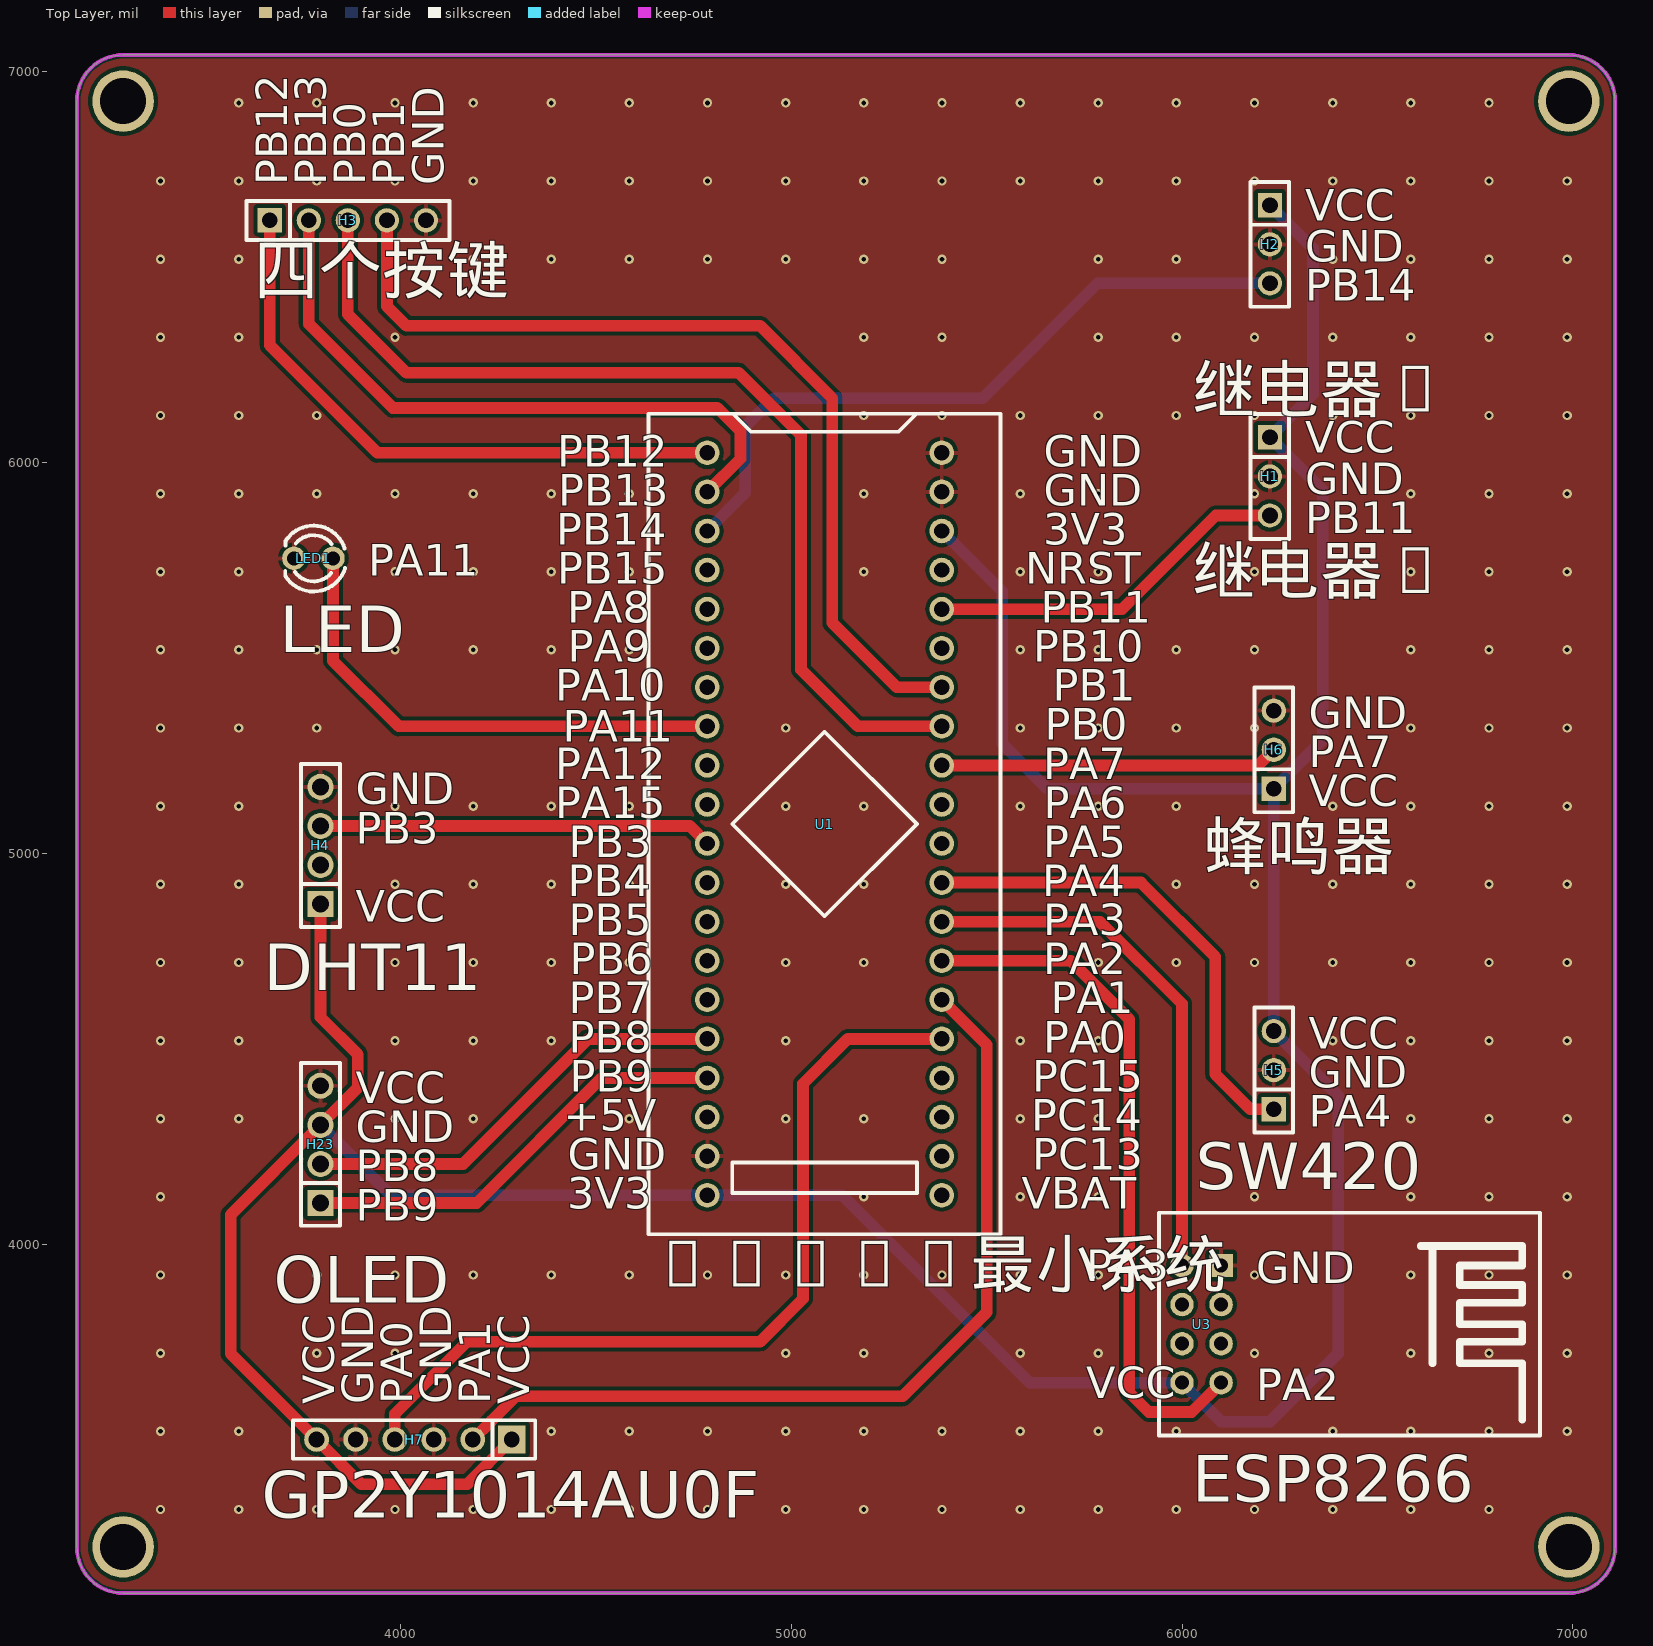
[diagram p0: Top Layer view]
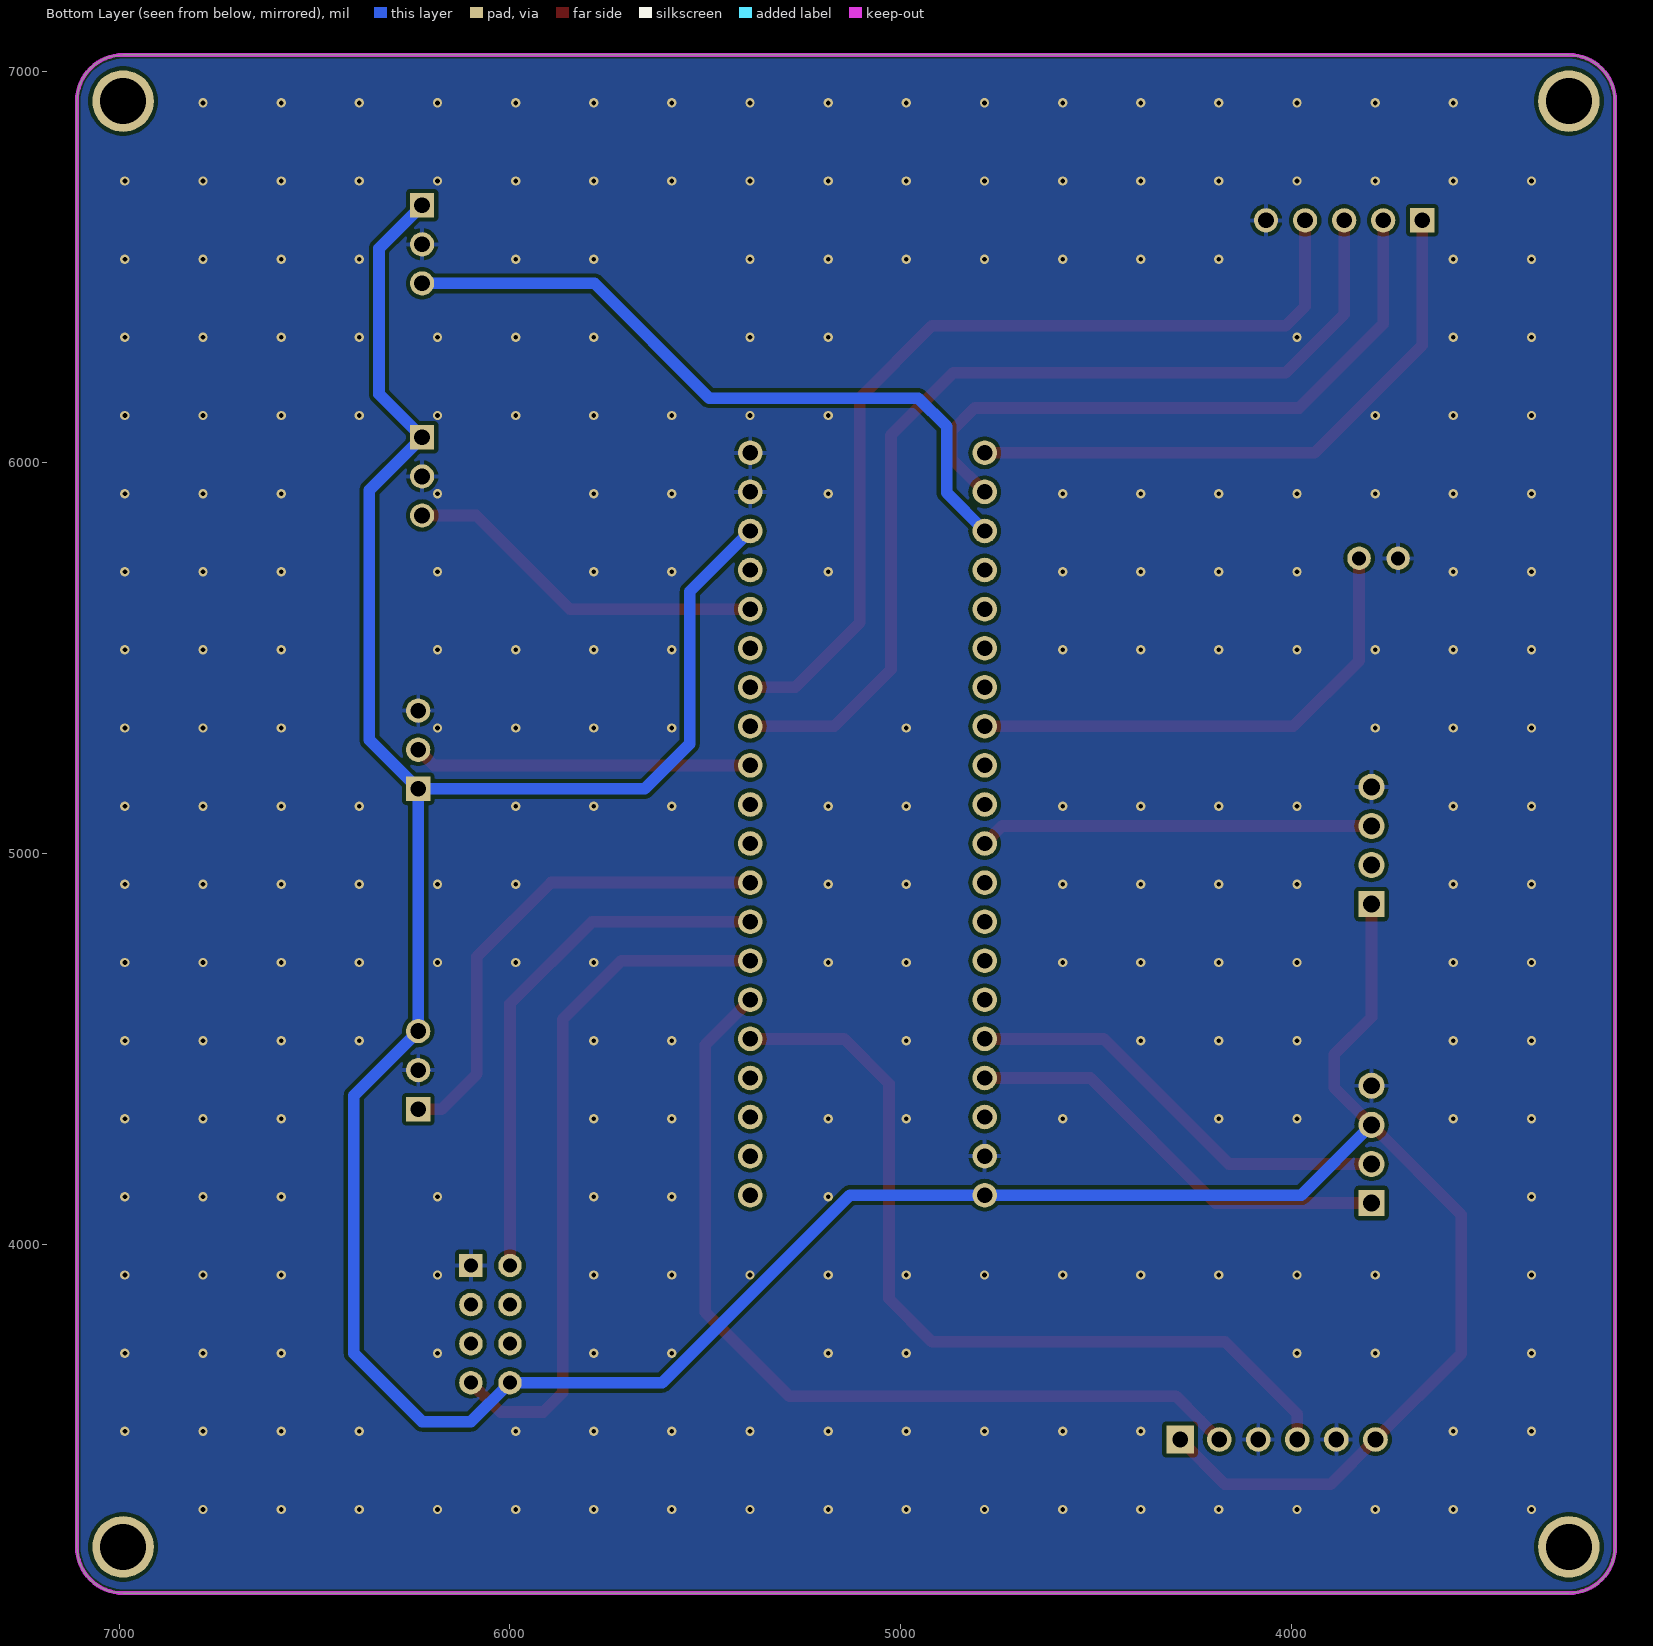
[diagram p1: Bottom Layer view, seen from below]
# Altium PCB MISC51358.pcbdoc
Units mil, origin at the board's own origin, x right, y up, seen from the top; angles counter-clockwise.
Board outline 3937.01 x 3937.01 mil, 2 copper layers (Top Layer, Bottom Layer), stack 62.206 mil thick; 11 components, 37 nets, 85 pads, 264 vias.

## Layer stack, top to bottom
Top Solder Mask Layer: solder mask 0.394, Dk 3.3
Top Layer: signal copper 1.379
Dielectric1: surface 59.449, FR4, Dk 4.5
Bottom Layer: signal copper 1.378
Bottom Solder Mask Layer: solder mask 0.394, Dk 3.3

## Board outline
6990.39,3106.5 ccw(c6990.39,3224.61) 7108.5,3224.61 7108.5,6925.39 ccw(c6990.39,6925.39) 6990.39,7043.5 3289.61,7043.5 ccw(c3289.61,6925.39) 3171.5,6925.39 3171.5,3224.61 ccw(c3289.61,3224.61) 3289.61,3106.5

## Design rules (kind name [scope] priority, off if disabled: settings)
BoardOutlineClearance copperThickness2oz_1 [All] p2 off: genericclearance=7.99 ignorepadtopadclearanceinfootprint=FALSE except(0: Arc-SplitContinuation Track-SplitContinuation SMDPad-SplitContinuation THPad-SplitContinuation Via-SplitContinuation Fill-SplitContinuation Region-SplitContinuation Poly-SplitContinuation Text-SplitContinuation Hole-SplitContinuation; 5.98: Arc-CutoutEdge Track-CutoutEdge SMDPad-CutoutEdge THPad-CutoutEdge Via-CutoutEdge Text-CutoutEdge; 6.89: Hole-OutlineEdge Hole-CutoutEdge; 10: Poly-OutlineEdge Poly-CutoutEdge; 11.81: Arc-OutlineEdge Track-OutlineEdge SMDPad-OutlineEdge THPad-OutlineEdge Via-OutlineEdge Fill-OutlineEdge Region-OutlineEdge Text-OutlineEdge Fill-CutoutEdge Region-CutoutEdge)
BoardOutlineClearance Plane_innerPlane_1 [All] p4 off: genericclearance=4.02 ignorepadtopadclearanceinfootprint=FALSE except(0: Arc-SplitContinuation Track-SplitContinuation SMDPad-SplitContinuation THPad-SplitContinuation Via-SplitContinuation Fill-SplitContinuation Region-SplitContinuation Poly-SplitContinuation Text-SplitContinuation Hole-SplitContinuation; 5.98: Arc-CutoutEdge Track-CutoutEdge SMDPad-CutoutEdge THPad-CutoutEdge Via-CutoutEdge Text-CutoutEdge; 6.89: Hole-OutlineEdge Hole-CutoutEdge; 10: Poly-OutlineEdge Poly-CutoutEdge; 11.81: Arc-OutlineEdge Track-OutlineEdge SMDPad-OutlineEdge THPad-OutlineEdge Via-OutlineEdge Fill-OutlineEdge Region-OutlineEdge Text-OutlineEdge Fill-CutoutEdge Region-CutoutEdge)
BoardOutlineClearance Copper_copperRegion_1 [All] p6 off: genericclearance=4.02 ignorepadtopadclearanceinfootprint=FALSE except(0: Arc-SplitContinuation Track-SplitContinuation SMDPad-SplitContinuation THPad-SplitContinuation Via-SplitContinuation Fill-SplitContinuation Region-SplitContinuation Poly-SplitContinuation Text-SplitContinuation Hole-SplitContinuation; 5.98: Arc-CutoutEdge Track-CutoutEdge SMDPad-CutoutEdge THPad-CutoutEdge Via-CutoutEdge Text-CutoutEdge; 6.89: Hole-OutlineEdge Hole-CutoutEdge; 10: Poly-OutlineEdge Poly-CutoutEdge; 11.81: Arc-OutlineEdge Track-OutlineEdge SMDPad-OutlineEdge THPad-OutlineEdge Via-OutlineEdge Fill-OutlineEdge Region-OutlineEdge Text-OutlineEdge Fill-CutoutEdge Region-CutoutEdge)
BoardOutlineClearance copperThickness1oz_1 [All] p8: genericclearance=4.02 ignorepadtopadclearanceinfootprint=FALSE except(0: Arc-SplitContinuation Track-SplitContinuation SMDPad-SplitContinuation THPad-SplitContinuation Via-SplitContinuation Fill-SplitContinuation Region-SplitContinuation Poly-SplitContinuation Text-SplitContinuation Hole-SplitContinuation; 5.98: Arc-CutoutEdge Track-CutoutEdge SMDPad-CutoutEdge THPad-CutoutEdge Via-CutoutEdge Text-CutoutEdge; 6.89: Hole-OutlineEdge Hole-CutoutEdge; 10: Poly-OutlineEdge Poly-CutoutEdge; 11.81: Arc-OutlineEdge Track-OutlineEdge SMDPad-OutlineEdge THPad-OutlineEdge Via-OutlineEdge Fill-OutlineEdge Region-OutlineEdge Text-OutlineEdge Fill-CutoutEdge Region-CutoutEdge)
Clearance copperThickness2oz [All] p1 off: gap=7.99 ignorepadtopadclearanceinfootprint=FALSE except(5.98: SMDPad-Track SMDPad-SMDPad THPad-Track SMDPad-THPad THPad-THPad Track-Via SMDPad-Via THPad-Via Via-Via Fill-SMDPad Region-SMDPad Fill-THPad Region-THPad Fill-Via Region-Via Fill-Fill Fill-Region Region-Region Arc-Track Arc-SMDPad Arc-THPad Arc-Via Fill-Arc Region-Arc Arc-Arc Text-Track SMDPad-Text Text-THPad Text-Via Fill-Text Region-Text Arc-Text Text-Text; 6.89: Hole-Track Hole-SMDPad Hole-THPad Hole-Via Fill-Hole Region-Hole Hole-Arc Hole-Text; 10: Poly-Track Poly-SMDPad Poly-THPad Poly-Via Poly-Fill Poly-Region Poly-Poly Poly-Arc Poly-Text Poly-Hole; 11.81: Fill-Track Region-Track)
Clearance Plane_innerPlane [All] p3 off: gap=4.02 ignorepadtopadclearanceinfootprint=FALSE except(5.98: SMDPad-Track SMDPad-SMDPad THPad-Track SMDPad-THPad THPad-THPad Track-Via SMDPad-Via THPad-Via Via-Via Fill-SMDPad Region-SMDPad Fill-THPad Region-THPad Fill-Via Region-Via Fill-Fill Fill-Region Region-Region Arc-Track Arc-SMDPad Arc-THPad Arc-Via Fill-Arc Region-Arc Arc-Arc Text-Track SMDPad-Text Text-THPad Text-Via Fill-Text Region-Text Arc-Text Text-Text; 6.89: Hole-Track Hole-SMDPad Hole-THPad Hole-Via Fill-Hole Region-Hole Hole-Arc Hole-Text; 10: Poly-Track Poly-SMDPad Poly-THPad Poly-Via Poly-Fill Poly-Region Poly-Poly Poly-Arc Poly-Text Poly-Hole; 11.81: Fill-Track Region-Track)
Clearance Copper_copperRegion [All] p5 off: gap=4.02 ignorepadtopadclearanceinfootprint=FALSE except(5.98: SMDPad-Track SMDPad-SMDPad THPad-Track SMDPad-THPad THPad-THPad Track-Via SMDPad-Via THPad-Via Via-Via Fill-SMDPad Region-SMDPad Fill-THPad Region-THPad Fill-Via Region-Via Fill-Fill Fill-Region Region-Region Arc-Track Arc-SMDPad Arc-THPad Arc-Via Fill-Arc Region-Arc Arc-Arc Text-Track SMDPad-Text Text-THPad Text-Via Fill-Text Region-Text Arc-Text Text-Text; 6.89: Hole-Track Hole-SMDPad Hole-THPad Hole-Via Fill-Hole Region-Hole Hole-Arc Hole-Text; 10: Poly-Track Poly-SMDPad Poly-THPad Poly-Via Poly-Fill Poly-Region Poly-Poly Poly-Arc Poly-Text Poly-Hole; 11.81: Fill-Track Region-Track)
Clearance copperThickness1oz [All] p7: gap=4.02 ignorepadtopadclearanceinfootprint=FALSE except(5.98: SMDPad-Track SMDPad-SMDPad THPad-Track SMDPad-THPad THPad-THPad Track-Via SMDPad-Via THPad-Via Via-Via Fill-SMDPad Region-SMDPad Fill-THPad Region-THPad Fill-Via Region-Via Fill-Fill Fill-Region Region-Region Arc-Track Arc-SMDPad Arc-THPad Arc-Via Fill-Arc Region-Arc Arc-Arc Text-Track SMDPad-Text Text-THPad Text-Via Fill-Text Region-Text Arc-Text Text-Text; 6.89: Hole-Track Hole-SMDPad Hole-THPad Hole-Via Fill-Hole Region-Hole Hole-Arc Hole-Text; 10: Poly-Track Poly-SMDPad Poly-THPad Poly-Via Poly-Fill Poly-Region Poly-Poly Poly-Arc Poly-Text Poly-Hole; 11.81: Fill-Track Region-Track)
DiffPairsRouting differentialPair [All] p1: maxlimit=6 minlimit=6 mostfreqgap=6 toplayer_minwidth=5 toplayer_prefwidth=10 toplayer_maxwidth=100 toplayer_mingap=6 toplayer_prefgap=6 toplayer_maxgap=6 bottomlayer_minwidth=5 bottomlayer_prefwidth=10 bottomlayer_maxwidth=100 bottomlayer_mingap=6 bottomlayer_prefgap=6 bottomlayer_maxgap=6 maxuncoupledlength=10
HoleToHoleClearance otherClearance [All] p1: gap=11.81 allowstackedmicrovias=TRUE
Length netLength [All] p1: minlimit=0 maxlimit=0
PasteMaskExpansion pasteMaskExpansion [All] p1: expansion=0
PlaneConnect innerPlane [All] p1: planeconnectstyle=Relief reliefexpansion=20 reliefentries=4 reliefconductorwidth=10 reliefairgap=10
PolygonConnect copperRegion [All] p1: connectstyle=Relief reliefconductorwidth=10 reliefentries=4 polygonreliefangle="90 Angle" airgapwidth=10 via.connectstyle=Relief via.reliefconductorwidth=10 via.reliefentries=4 via.polygonreliefangle="90 Angle" via.airgapwidth=10
RoutingVias viaSize [All] p1: holewidth=12.01 width=24.02 viastyle="Through Hole" minholewidth=11.81 minwidth=19.68 maxholewidth=248.03 maxwidth=393.7
SolderMaskExpansion solderMaskExpansion [IsVia] p1: expansion=-1000 istentingtop=TRUE
SolderMaskExpansion solderMaskExpansion [All] p2: expansion=2.01 istentingtop=FALSE
Width copperThickness2oz_2 [All] p1 off: maxlimit=100 minlimit=8 preferedwidth=10
Width copperThickness1oz_2 [All] p2: maxlimit=100 minlimit=5 preferedwidth=30

## Components (designator, comment, footprint, x,y, rotation, side; value= is the part's Value field where it differs from the comment)
H1 "" HDR-TH_3P-P2.54-V-F 6225,5964.59 r270 top
H2 "" HDR-TH_3P-P2.54-V-F 6225,6558.68 r270 top
H3 "" HDR-TH_5P-P2.54-V-F 3865,6620 r0 top
H4 "" HDR-TH_4P-P2.54-V-F 3795,5020 r90 top
H5 "" HDR-TH_3P-P2.54-V-F 6234.84,4445 r90 top
H6 "" HDR-TH_3P-P2.54-V-F 6234.84,5265.03 r90 top
H7 "" HDR-TH_6P-P2.54-V-F 4034.9,3499.62 r180 top
H23 "" HDR-TH_4P-P2.54-V-F 3795,4255 r90 top
LED1 "" LED_TH-3mm 3776.87,5755 r180 top
U1 "STM32F103C8T6-Card" CONN-TH_L53.3-W22.9_STM32F103C8T6-CARD 5085,5075 r270 top
U3 "ESP8266-01S" WIFIM-TH_ESP8266-01S 6050,3795 r270 top

## Footprints (in the part's own frame and the unit in brackets; to place one, negate y for a bottom-side part, rotate by r counter-clockwise, add the part's x,y. Pads: shape width x height; smd on the part's side, far side on the other; paste and mask are expansions set on the pad)
CONN-TH_L53.3-W22.9_STM32F103C8T6-CARD [mm]
  round 1.6 hole 1: 1(-24.13,-7.62) 2(-21.59,-7.62) 3(-19.05,-7.62) 4(-16.51,-7.62) 5(-13.97,-7.62) 6(-11.43,-7.62) 7(-8.89,-7.62) 8(-6.35,-7.62) 9(-3.81,-7.62) 10(-1.27,-7.62) 11(1.27,-7.62) 12(3.81,-7.62) 13(6.35,-7.62) 14(8.89,-7.62) 15(11.43,-7.62) 16(13.97,-7.62) 17(16.51,-7.62) 18(19.05,-7.62) 19(21.59,-7.62) 20(24.13,-7.62) 21(24.13,7.62) 22(21.59,7.62) 23(19.05,7.62) 24(16.51,7.62) 25(13.97,7.62) 26(11.43,7.62) 27(8.89,7.62) 28(6.35,7.62) 29(3.81,7.62) 30(1.27,7.62) 31(-1.27,7.62) 32(-3.81,7.62) 33(-6.35,7.62) 34(-8.89,7.62) 35(-11.43,7.62) 36(-13.97,7.62) 37(-16.51,7.62) 38(-19.05,7.62) 39(-21.59,7.62) 40(-24.13,7.62)
  silkscreen extent -26.67,-11.43 26.67,11.43
HDR-TH_3P-P2.54-V-F [mil]
  rect 62x62 hole 40.16: 1(-100,0)
  round 62 hole 40.16: 2(0,0) 3(100,0)
  silkscreen extent -160,-49 160,49
HDR-TH_4P-P2.54-V-F [mm]
  rect 1.7x1.7 hole 1.1: 1(-3.81,0)
  round 1.7 hole 1.1: 2(-1.27,0) 3(1.27,0) 4(3.81,0)
  silkscreen extent -5.29,-1.27 5.29,1.27
HDR-TH_5P-P2.54-V-F [mil]
  rect 62x62 hole 40.16: 1(-200,0)
  round 62 hole 40.16: 2(-100,0) 3(0,0) 4(100,0) 5(200,0)
  silkscreen extent -260,-50 260,50
HDR-TH_6P-P2.54-V-F [mm]
  rect 1.8x1.8 hole 1.02: 1(-6.35,0)
  round 1.6 hole 1.02: 2(-3.81,0) 3(-1.27,0) 4(1.27,0) 5(3.81,0) 6(6.35,0)
  silkscreen extent -7.87,-1.25 7.87,1.25
LED_TH-3mm [mil]
  round 60 hole 36 paste+0 mask+2: 1(-50,0) 2(50,0)
  silkscreen extent -81,-84 72,85
WIFIM-TH_ESP8266-01S [mil]
  rect 60x60 hole 36 paste+0 mask+1.97: 1(-150,50)
  round 60 hole 36 paste+0 mask+1.97: 2(-50,50) 3(50,50) 4(150,50) 5(-150,-50) 6(-50,-50) 7(50,-50) 8(150,-50)
  silkscreen extent -285,-109 285,866

## Free pads (board coordinates)
  round 157.48 hole 118.11: 1(3289.61,6925.39) 1(3289.61,3224.61) 1(6990.39,6925.39) 1(6990.39,3224.61)

## Via types
v1: diameter 24.02, hole 12, Top Layer to Bottom Layer, 264 vias

## Nets (pads, with @x,y where several pads share a name; then routed paths per layer and width w, separated by ;. In a path a pad name is that pad's centre, name@x,y a point inside that pad or via, vN(x,y) a via of type N, cw(c..) or ccw(c..) an arc to the next point about the centre after c; other vN are vias at no path point)
+5V: U1.18
GND: H1.2 H2.2 H3.5 H4.4 H5.2 H6.3 H7.3 H7.5 H23.4 LED1.2 U1.19 U1.39 U1.40 U3.1
  other v1: 3385.6,3320.6 3585.6,3320.6 3785.6,3320.6 3985.6,3320.6 4185.6,3320.6 4385.6,3320.6 4585.6,3320.6 4785.6,3320.6 4985.6,3320.6 5185.6,3320.6 5385.6,3320.6 5585.6,3320.6 5785.6,3320.6 5985.6,3320.6 6185.6,3320.6 6385.6,3320.6 6585.6,3320.6 6785.6,3320.6 3385.6,3520.6 3585.6,3520.6 4385.6,3520.6 4585.6,3520.6 4785.6,3520.6 4985.6,3520.6 5185.6,3520.6 5385.6,3520.6 5585.6,3520.6 5785.6,3520.6 5985.6,3520.6 6385.6,3520.6 6585.6,3520.6 6785.6,3520.6 6985.6,3520.6 3385.6,3720.6 3785.6,3720.6 3985.6,3720.6 4985.6,3720.6 5185.6,3720.6 5585.6,3720.6 5785.6,3720.6 6185.6,3720.6 6585.6,3720.6 6785.6,3720.6 6985.6,3720.6 3385.6,3920.6 3785.6,3920.6 3985.6,3920.6 4185.6,3920.6 4385.6,3920.6 4585.6,3920.6 4785.6,3920.6 4985.6,3920.6 5185.6,3920.6 5385.6,3920.6 5585.6,3920.6 5785.6,3920.6 6185.6,3920.6 6585.6,3920.6 6785.6,3920.6 6985.6,3920.6 3385.6,4120.6 5185.6,4120.6 5585.6,4120.6 5785.6,4120.6 6185.6,4120.6 6585.6,4120.6 6785.6,4120.6 6985.6,4120.6 3385.6,4320.6 3585.6,4320.6 3985.6,4320.6 4185.6,4320.6 4585.6,4320.6 4985.6,4320.6 5185.6,4320.6 5585.6,4320.6 5785.6,4320.6 6585.6,4320.6 6785.6,4320.6 6985.6,4320.6 3385.6,4520.6 3585.6,4520.6 3985.6,4520.6 4185.6,4520.6 4385.6,4520.6 4985.6,4520.6 5585.6,4520.6 5785.6,4520.6 6385.6,4520.6 6585.6,4520.6 6785.6,4520.6 6985.6,4520.6 3385.6,4720.6 3585.6,4720.6 3985.6,4720.6 4185.6,4720.6 4385.6,4720.6 4585.6,4720.6 4985.6,4720.6 5185.6,4720.6 5785.6,4720.6 5985.6,4720.6 6185.6,4720.6 6385.6,4720.6 6585.6,4720.6 6785.6,4720.6 6985.6,4720.6 3385.6,4920.6 3585.6,4920.6 3985.6,4920.6 4185.6,4920.6 4385.6,4920.6 4585.6,4920.6 4985.6,4920.6 5185.6,4920.6 5985.6,4920.6 6185.6,4920.6 6385.6,4920.6 6585.6,4920.6 6785.6,4920.6 6985.6,4920.6 3385.6,5120.6 3585.6,5120.6 3985.6,5120.6 4185.6,5120.6 4385.6,5120.6 4585.6,5120.6 4985.6,5120.6 5185.6,5120.6 5585.6,5120.6 5785.6,5120.6 5985.6,5120.6 6385.6,5120.6 6585.6,5120.6 6785.6,5120.6 6985.6,5120.6 3385.6,5320.6 3585.6,5320.6 3785.6,5320.6 4985.6,5320.6 5585.6,5320.6 5785.6,5320.6 5985.6,5320.6 6185.6,5320.6 6585.6,5320.6 6785.6,5320.6 6985.6,5320.6 3385.6,5520.6 3585.6,5520.6 3785.6,5520.6 3985.6,5520.6 4185.6,5520.6 4385.6,5520.6 4585.6,5520.6 5585.6,5520.6 5785.6,5520.6 5985.6,5520.6 6185.6,5520.6 6585.6,5520.6 6785.6,5520.6 6985.6,5520.6 3385.6,5720.6 3585.6,5720.6 3985.6,5720.6 4185.6,5720.6 4385.6,5720.6 4585.6,5720.6 5185.6,5720.6 5585.6,5720.6 5785.6,5720.6 6185.6,5720.6 6585.6,5720.6 6785.6,5720.6 6985.6,5720.6 3385.6,5920.6 3585.6,5920.6 3785.6,5920.6 3985.6,5920.6 4185.6,5920.6 4385.6,5920.6 4585.6,5920.6 5185.6,5920.6 5585.6,5920.6 5785.6,5920.6 6185.6,5920.6 6585.6,5920.6 6785.6,5920.6 6985.6,5920.6 3385.6,6120.6 3585.6,6120.6 3785.6,6120.6 5185.6,6120.6 5385.6,6120.6 5585.6,6120.6 5785.6,6120.6 5985.6,6120.6 6185.6,6120.6 6385.6,6120.6 6585.6,6120.6 6785.6,6120.6 6985.6,6120.6 3385.6,6320.6 3585.6,6320.6 3985.6,6320.6 5185.6,6320.6 5385.6,6320.6 5785.6,6320.6 5985.6,6320.6 6185.6,6320.6 6385.6,6320.6 6585.6,6320.6 6785.6,6320.6 6985.6,6320.6 3385.6,6520.6 3585.6,6520.6 4185.6,6520.6 4385.6,6520.6 4585.6,6520.6 4785.6,6520.6 4985.6,6520.6 5185.6,6520.6 5385.6,6520.6 5785.6,6520.6 5985.6,6520.6 6385.6,6520.6 6585.6,6520.6 6785.6,6520.6 6985.6,6520.6 3385.6,6720.6 3585.6,6720.6 3785.6,6720.6 3985.6,6720.6 4185.6,6720.6 4385.6,6720.6 4585.6,6720.6 4785.6,6720.6 4985.6,6720.6 5185.6,6720.6 5385.6,6720.6 5585.6,6720.6 5785.6,6720.6 5985.6,6720.6 6185.6,6720.6 6385.6,6720.6 6585.6,6720.6 6785.6,6720.6 6985.6,6720.6 3585.6,6920.6 3785.6,6920.6 3985.6,6920.6 4185.6,6920.6 4385.6,6920.6 4585.6,6920.6 4785.6,6920.6 4985.6,6920.6 5185.6,6920.6 5385.6,6920.6 5585.6,6920.6 5785.6,6920.6 5985.6,6920.6 6185.6,6920.6 6385.6,6920.6 6585.6,6920.6 6785.6,6920.6
NRST: U1.37
PA0: H7.4 U1.25 | length 2185.2
  Top Layer w30: H7.4 3984.9,3564.9 4170,3750 4920,3750 5030,3860 5030,4410 5145,4525 U1.25
PA1: H7.2 U1.26 | length 2297.6
  Top Layer w30: H7.2 4232.08,3546.8 cw(c4249.47,3535.06) 4237.72,3552.45 4295.27,3610 5285,3610 5500,3825 5500,4510 U1.26
PA2: U1.27 U3.4 | length 1783.9
  Top Layer w30: U1.27 5715,4725 5865,4575 5865,3620 5915,3570 6025,3570 U3.4
PA3: U1.28 U3.5 | length 1372
  Top Layer w30: U1.28 5790,4825 6000,4615 U3.5
PA4: H5.1 U1.29 | length 1265.8
  Top Layer w30: U1.29 5895,4925 6085,4735 6085,4435 6175,4345 H5.1
PA5: U1.30
PA6: U1.31
PA7: H6.2 U1.32 | length 866.4
  Top Layer w30: U1.32 6194.81,5225 H6.2
PA8: U1.5
PA9: U1.6
PA10: U1.7
PA11: LED1.1 U1.8 | length 1289.6
  Top Layer w30: LED1.1 3826.87,5493.13 3995,5325 U1.8
PA12: U1.9
PA15: U1.10
PB0: H3.3 U1.33 | length 2548.5
  Top Layer w30: H3.3 3865,6380 4015,6230 4865,6230 5025,6070 5025,5470 5170,5325 U1.33
PB1: H3.4 U1.34 | length 2380.7
  Top Layer w30: H3.4 3965,6400 4015,6350 4920,6350 5105,6165 5105,5590 5270,5425 U1.34
PB3: H4.3 U1.11 | length 1008.6
  Top Layer w30: H4.3 4740,5070 U1.11
PB4: U1.12
PB5: U1.13
PB6: U1.14
PB7: U1.15
PB8: H23.2 U1.16 | length 1122.5
  Top Layer w30: H23.2 4160,4205 4480,4525 U1.16
PB9: H23.1 U1.17 | length 1122.5
  Top Layer w30: H23.1 4195,4105 4515,4425 U1.17
PB10: U1.35
PB11: H1.3 U1.36 | length 939.2
  Top Layer w30: U1.36 5846.47,5625 6086.06,5864.59 H1.3
PB12: H3.1 U1.1 | length 1553.9
  Top Layer w30: H3.1 3665,6300 3940,6025 U1.1
PB13: H3.2 U1.2 | length 1674.1
  Top Layer w30: H3.2 3765,6355 3980,6140 4810,6140 4870,6080 4870,6010 U1.2
PB14: H2.3 U1.3 | length 1802.1
  Bottom Layer w30: U1.3 4882.48,5922.48 4882.48,6092.48 4955,6165 5490,6165 5783.68,6458.68 H2.3
PB15: U1.4
PC13: U1.22
PC14: U1.23
PC15: U1.24
VBAT: U1.21
VCC: H1.1 H2.1 H4.1 H5.3 H6.1 H7.1 H7.6 H23.3 U1.20 U1.38 U3.8 | length 9780.3
  Top Layer w30: H4.1 3795,4580.24 3890,4485.24 3890,4400 H23.3 3565,4075 3565,3719.52 H7.6 3899.52,3385 4170.27,3385 H7.1
  Bottom Layer w30: H23.3 3975,4125 U1.20 5130,4125 5610,3645 U3.8 6100,3545 6225,3545 6400,3720 6400,4379.84 H5.3 H6.1 ; U1.38 5540,5670 5540,5280 5654.97,5165.03 H6.1 ; H2.1 6335,6548.68 6335,6174.59 H1.1 6360,5929.59 6360,5290.19 H6.1
pads on no net: H4.2 U3.2 U3.3 U3.6 U3.7

## Polygon pours and split planes (outlines as drawn)
GND on Bottom Layer (solid, remove dead copper, pour order 2): 3100,7165 3100,3000 7275,3000 7275,7165
GND on Top Layer (solid, remove dead copper, pour order 0): 3000,7145 3000,3075 7385,3075 7385,7145

## Keep-outs
Board Outline Layer:
  the board outline again, w10

## Silkscreen, mask and mechanical layers (free items; w line width, h text height)
Top Silkscreen Layer:
  text "PB12" at 3710,6709.9 h80 r90
  text "PB13" at 3810,6709.9 h80 r90
  text "PB0" at 3910,6709.9 h80 r90
  text "PB1" at 4010,6709.9 h80 r90
  text "GND" at 4110,6709.9 h80 r90
  text "VCC" at 6314.9,6618.68 h80
  text "GND" at 6314.9,6513.68 h80
  text "四个按键" at 3625,6435 h120
  text "PB14" at 6314.9,6413.68 h80
  text "继电器2" at 6025.16,6130 h120
  text "VCC" at 6314.9,6024.59 h80
  text "PB12" at 4400.64,5990 h80
  text "GND" at 5646.65,5990 h80
  text "GND" at 6314.9,5919.59 h80
  text "PB13" at 4403.85,5890 h80
  text "GND" at 5646.65,5890 h80
  text "PB11" at 6314.9,5819.59 h80
  text "PB14" at 4398.34,5790 h80
  text "3V3" at 5644.45,5790 h80
  text "PA11" at 3916.77,5710 h80
  text "PB15" at 4400.64,5690 h80
  text "NRST" at 5598.65,5690 h80
  text "继电器1" at 6025,5665 h120
  text "PA8" at 4426.24,5590 h80
  text "PB11" at 5639.05,5590 h80
  text "LED" at 3690.36,5515 h120
  text "PA9" at 4428.44,5490 h80
  text "PB10" at 5618.85,5490 h80
  text "PA10" at 4396.14,5390 h80
  text "PB1" at 5669.15,5390 h80
  text "GND" at 6324.74,5320.03 h80
  text "PB0" at 5648.95,5290 h80
  text "PA11" at 4414.55,5285 h80
  text "PA7" at 6324.74,5220.03 h80
  text "PA12" at 4396.14,5190 h80
  text "PA7" at 5644.45,5190 h80
  text "GND" at 3884.9,5125 h80
  text "VCC" at 6324.74,5120.03 h80
  text "PA15" at 4396.14,5090 h80
  text "PA6" at 5646.65,5090 h80
  text "PB3" at 3884.9,5025 h80
  text "PB3" at 4430.74,4990 h80
  text "PA5" at 5644.45,4990 h80
  text "蜂鸣器" at 6054.68,4960 h120
  text "PB4" at 4428.44,4890 h80
  text "PA4" at 5642.15,4890 h80
  text "VCC" at 3884.9,4825 h80
  text "PB5" at 4430.74,4790 h80
  text "PA3" at 5644.45,4790 h80
  text "PB6" at 4432.94,4690 h80
  text "PA2" at 5644.45,4690 h80
  text "DHT11" at 3650.09,4650 h120
  text "PB7" at 4430.74,4590 h80
  text "PA1" at 5664.65,4590 h80
  text "VCC" at 6324.74,4500 h80
  text "PB8" at 4430.74,4490 h80
  text "PA0" at 5644.45,4490 h80
  text "GND" at 6324.74,4400 h80
  text "PB9" at 4432.94,4390 h80
  text "PC15" at 5616.55,4390 h80
  text "VCC" at 3884.9,4360 h80
  text "PA4" at 6324.74,4300 h80
  text "+5V" at 4417.24,4290 h80
  text "PC14" at 5614.25,4290 h80
  text "GND" at 3884.9,4260 h80
  text "GND" at 4428.44,4190 h80
  text "PC13" at 5616.55,4190 h80
  text "PB8" at 3884.9,4160 h80
  text "SW420" at 6035,4140 h120
  text "3V3" at 4426.24,4090 h80
  text "VBAT" at 5589.65,4090 h80
  text "PB9" at 3884.9,4060 h80
  text "PA3" at 5754.9,3905 h80
  text "GND" at 6189.9,3900 h80
  text "STM32最小系统" at 4640,3890 h120
  text "OLED" at 3675.18,3850 h120
  text "VCC" at 5754.9,3605 h80
  text "PA2" at 6189.9,3600 h80
  text "VCC" at 3829.9,3589.52 h80 r90
  text "GND" at 3929.9,3589.52 h80 r90
  text "PA0" at 4029.9,3589.52 h80 r90
  text "GND" at 4129.9,3589.52 h80 r90
  text "PA1" at 4229.9,3589.52 h80 r90
  text "VCC" at 4329.9,3589.52 h80 r90
  text "ESP8266" at 6026.3,3340 h120
  text "GP2Y1014AU0F" at 3645,3300 h120